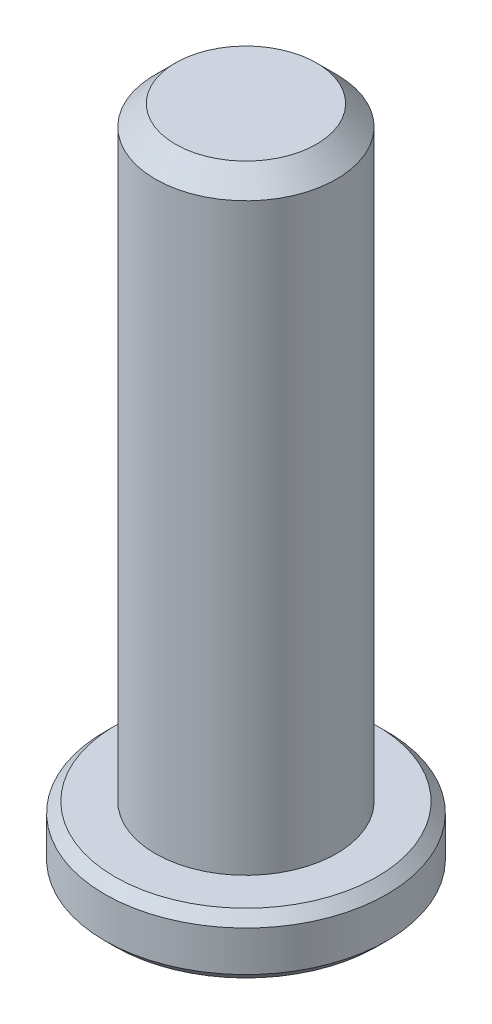
SolidWorks part; units mm, degrees
material "普通碳钢"
ref_plane "Front Plane" through (0, 0, 0) normal (0, 0, 1) x (1, 0, 0)
ref_plane "Top Plane" through (0, 0, 0) normal (0, 1, 0) x (1, 0, 0)
ref_plane "Right Plane" through (0, 0, 0) normal (1, 0, 0) x (0, 0, -1)
sketch "Sketch1" plane through (0, 0, 0) normal (0, 1, 0) x (1, 0, 0)
  circle A0 centre (0, 0) radius 7
  dimension "D1" = 14
extrude "Boss-Extrude1" add sketch "Sketch1" along normal blind 3
sketch "Sketch2" plane through (0, 3, 0) normal (0, 1, 0) x (1, 0, 0)
  circle A0 centre (0, 0) radius 4.5
  dimension "D1" = 9
extrude "Boss-Extrude2" add sketch "Sketch2" along normal blind 30
chamfer "Chamfer1" distance 1 angle 45 1 edges at (0, 33, 4.5)
chamfer "Chamfer2" distance 0.5 angle 45 2 edges at (0, 0, 7) (0, 3, 7)
